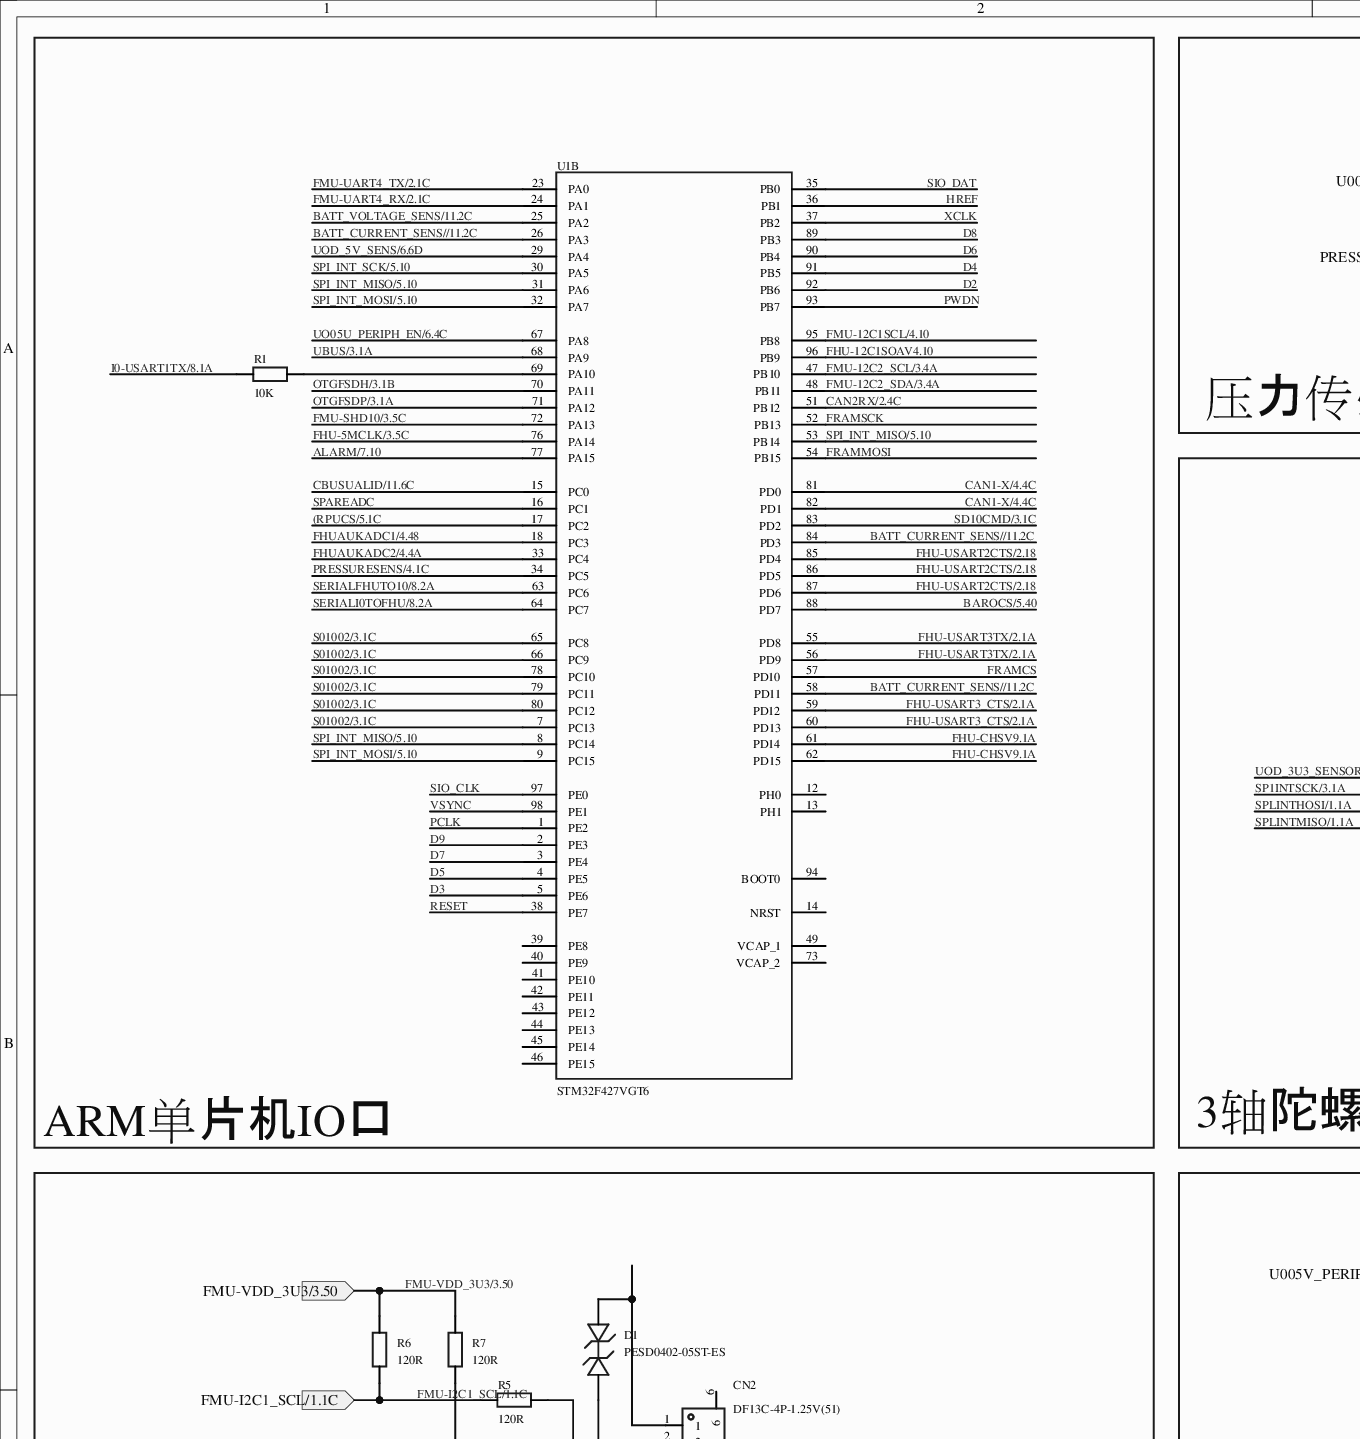
[diagram p0: MISC50255-3.schdoc, top left]
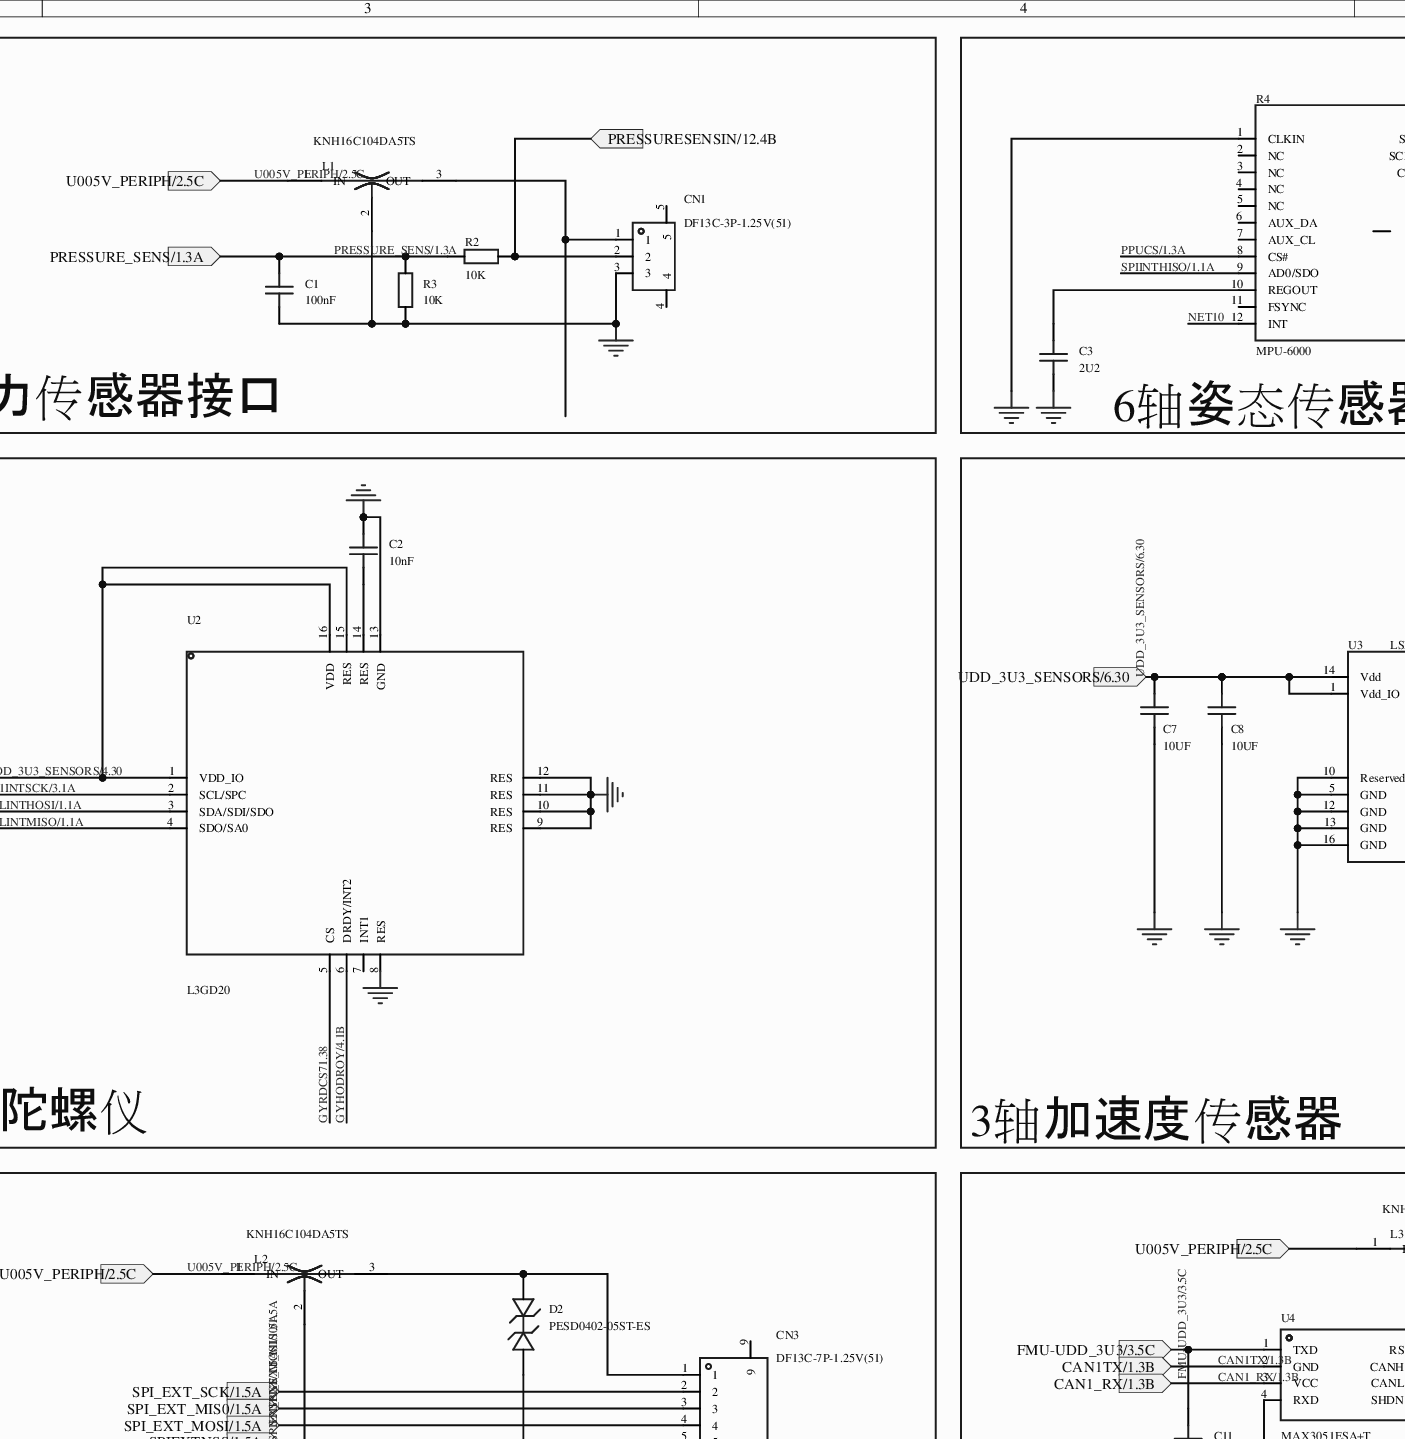
[diagram p1: MISC50255-3.schdoc, top middle]
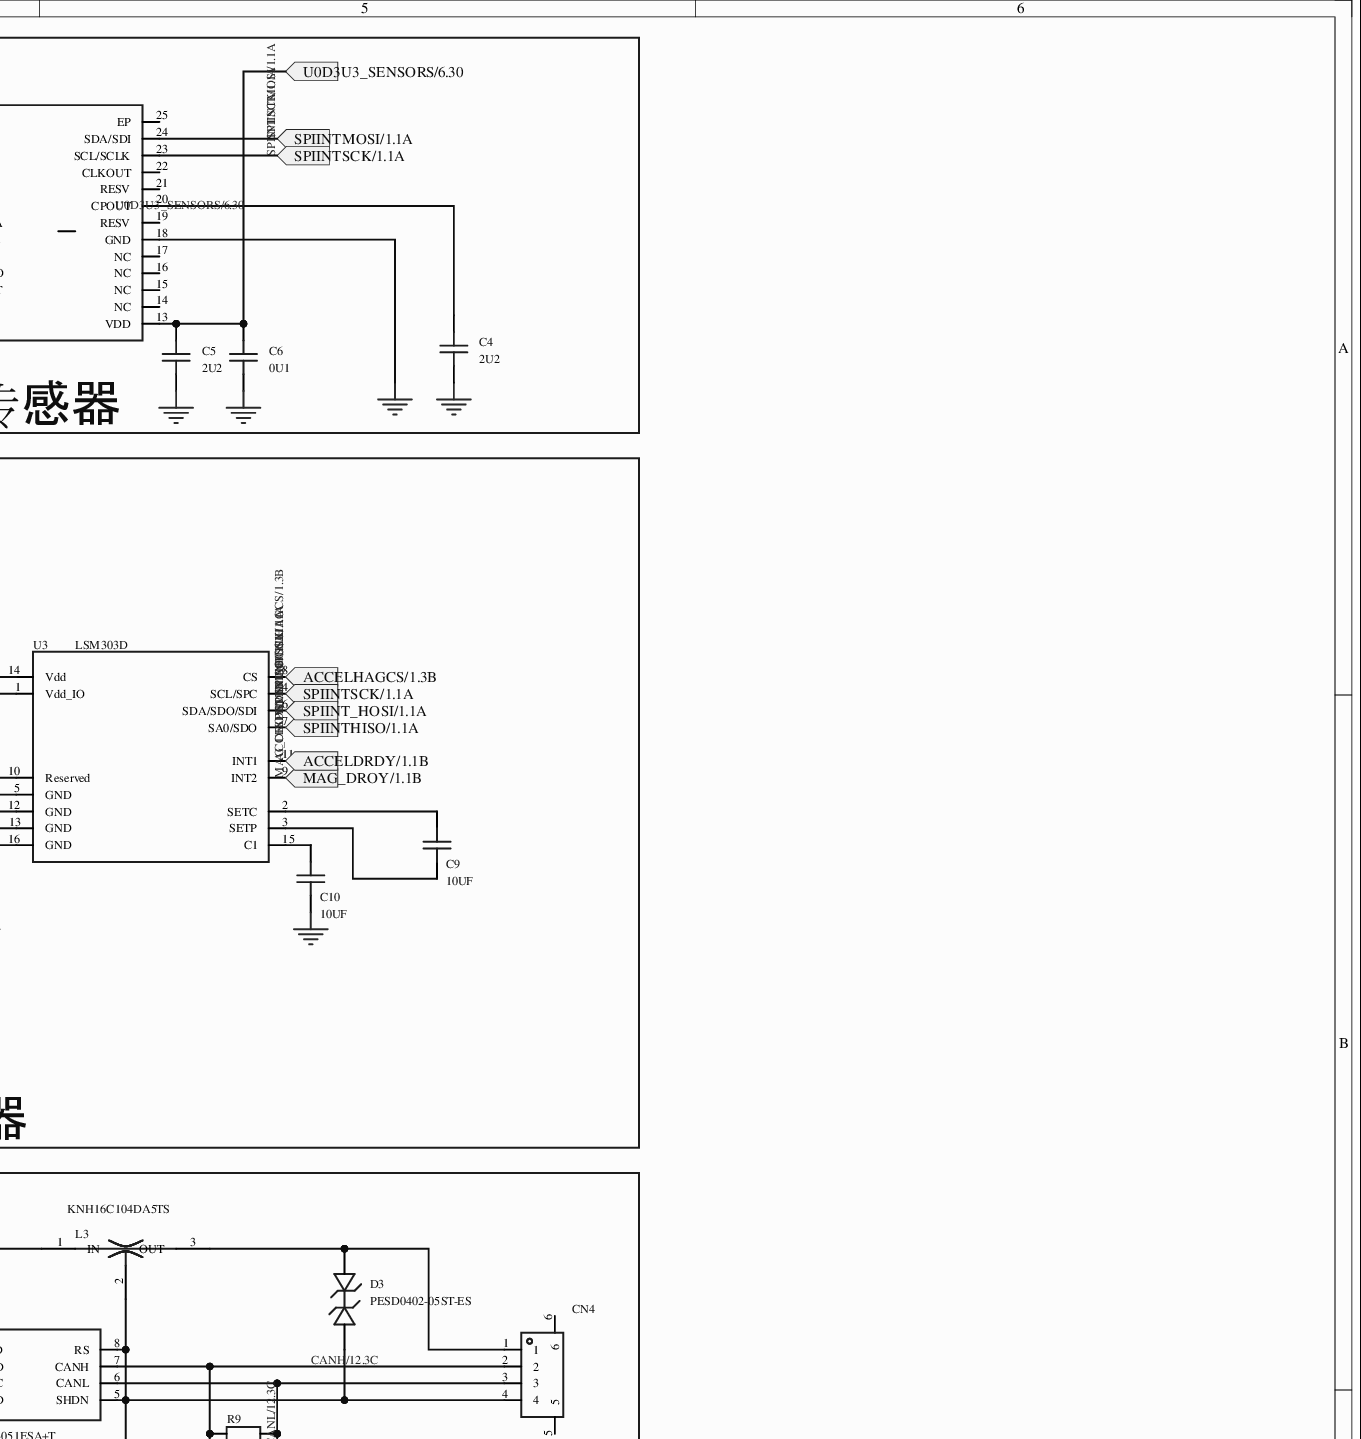
[diagram p2: MISC50255-3.schdoc, top right]
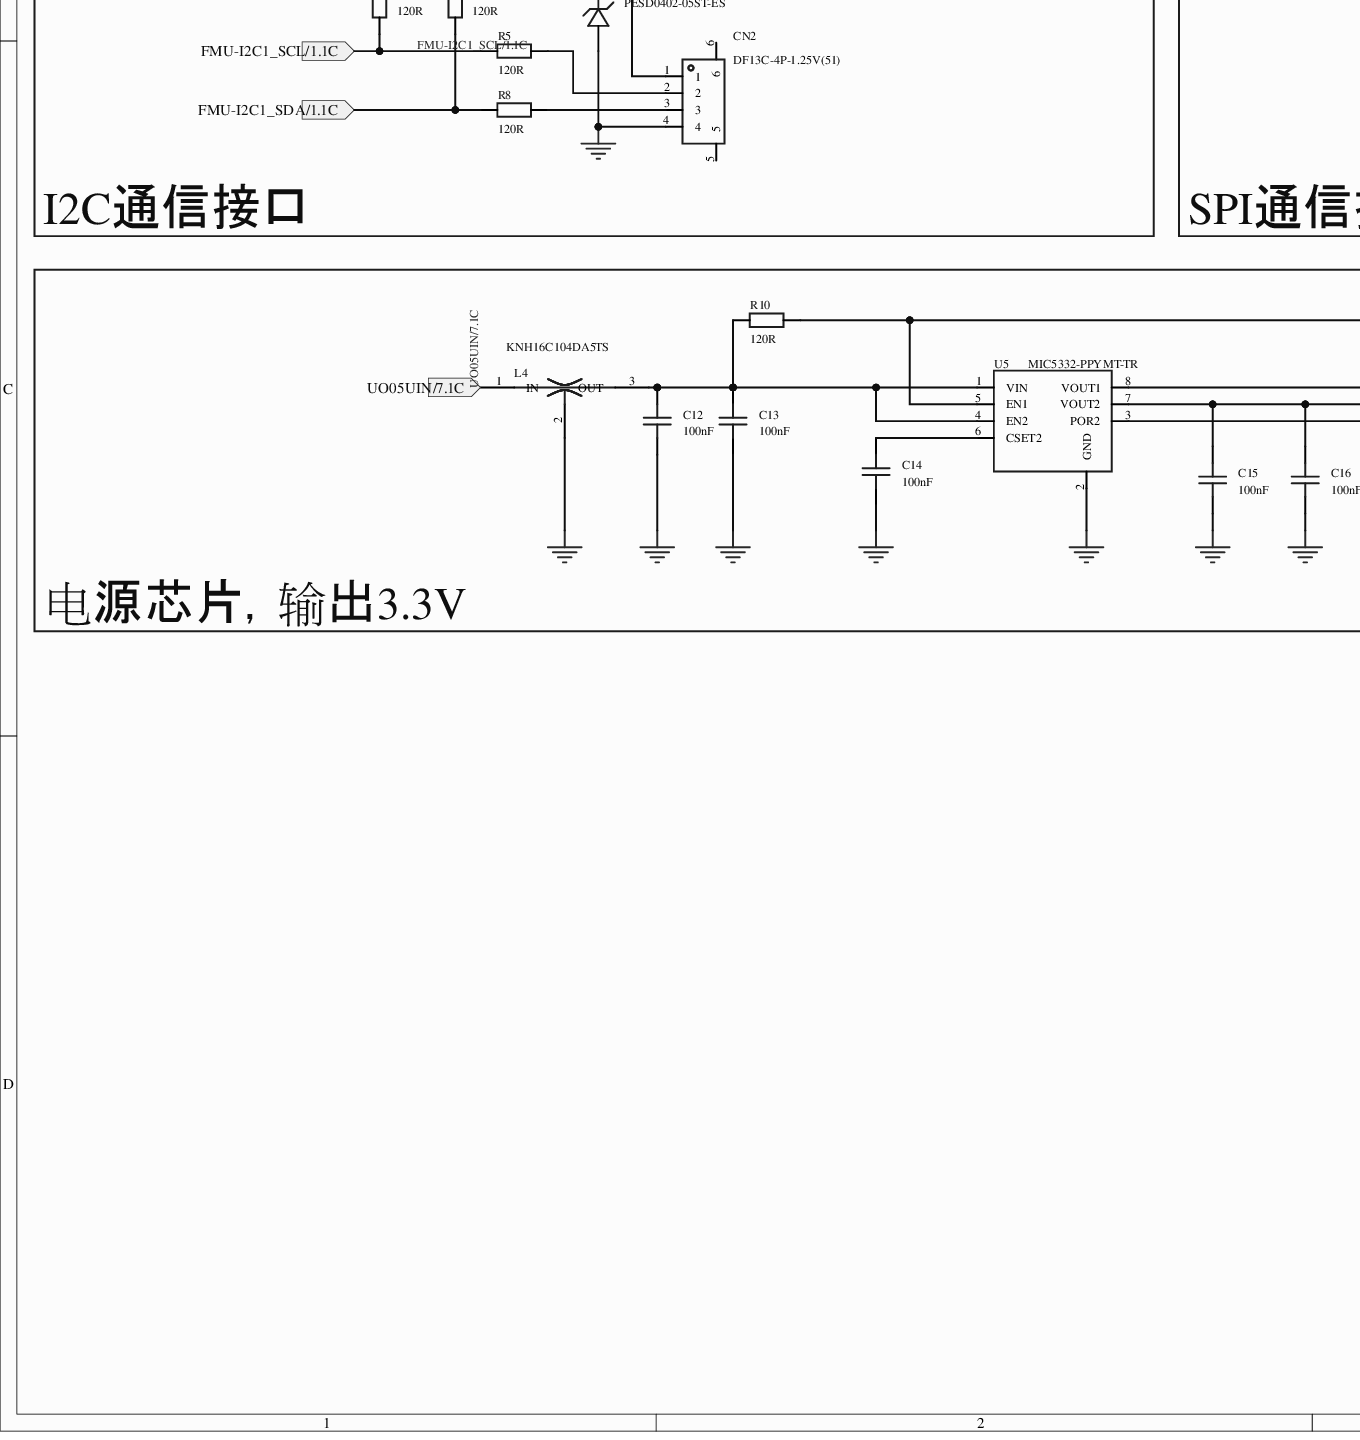
[diagram p3: MISC50255-3.schdoc, bottom left]
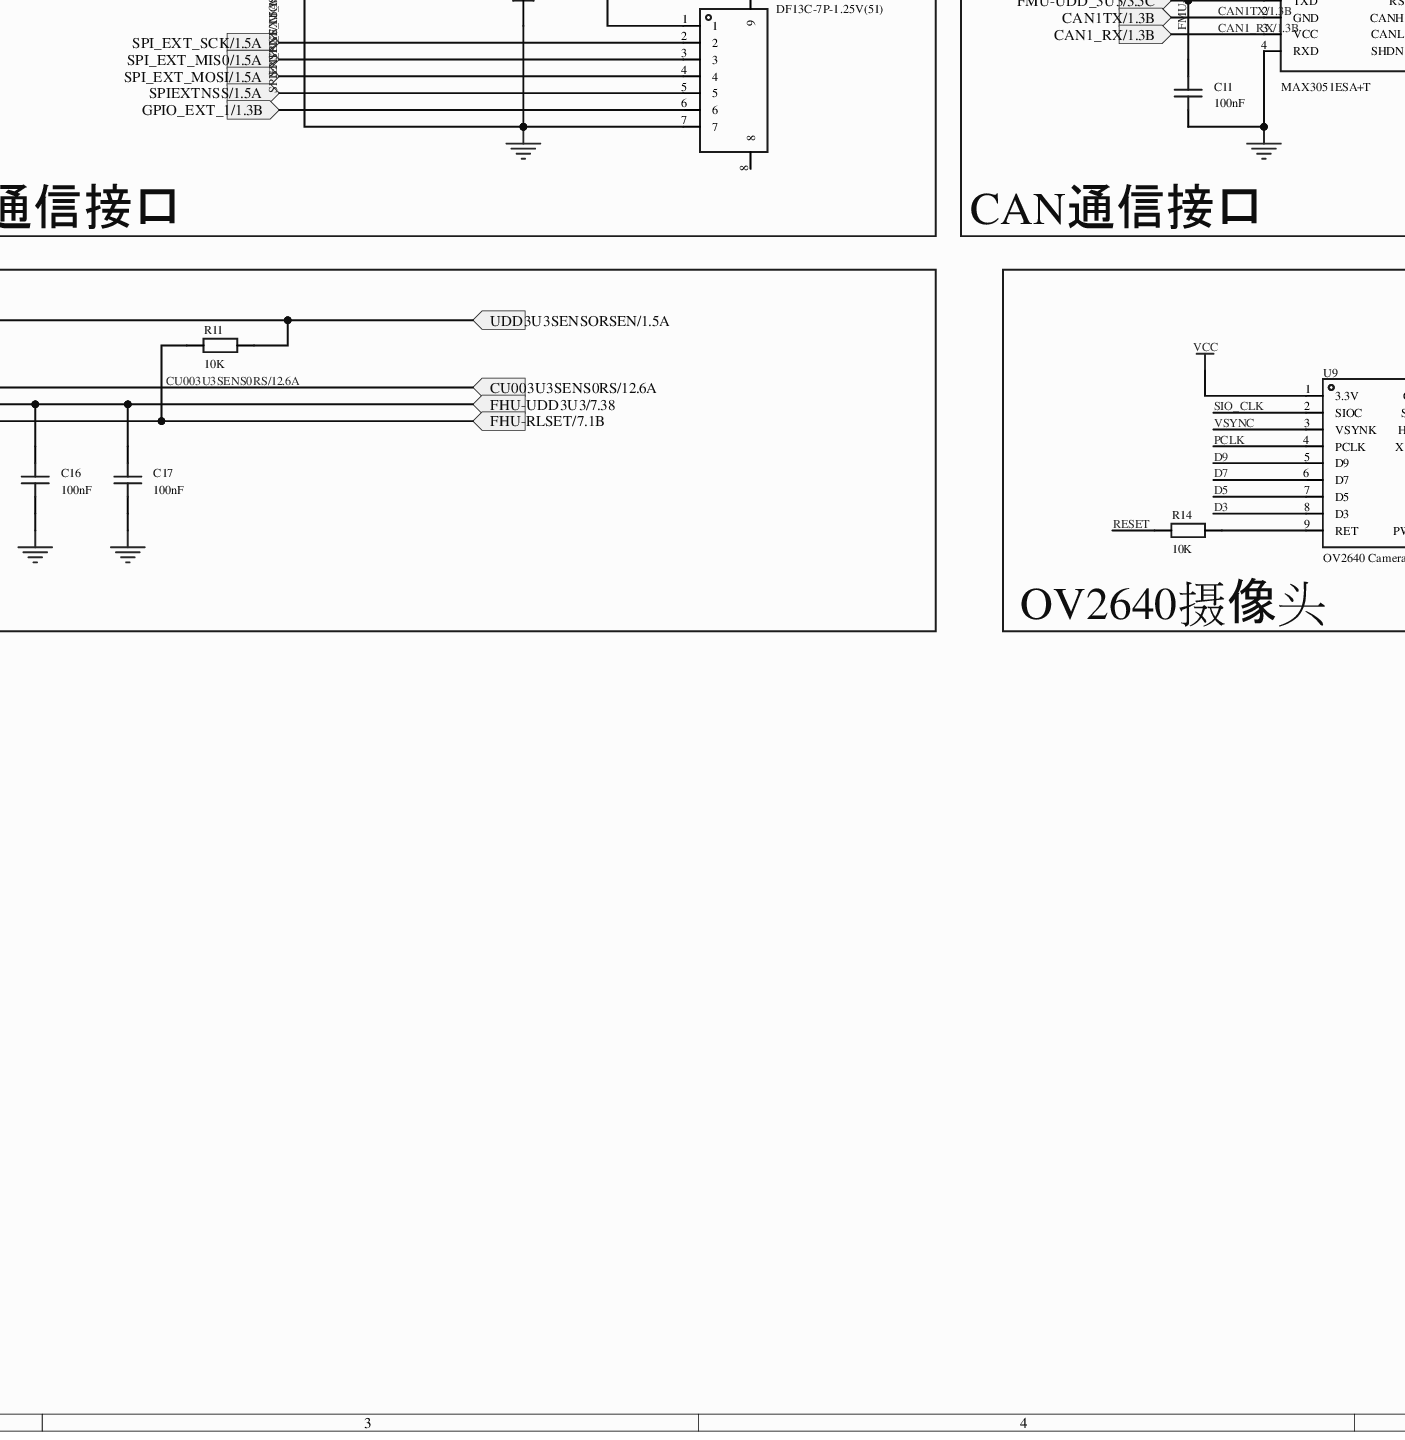
[diagram p4: MISC50255-3.schdoc, bottom middle]
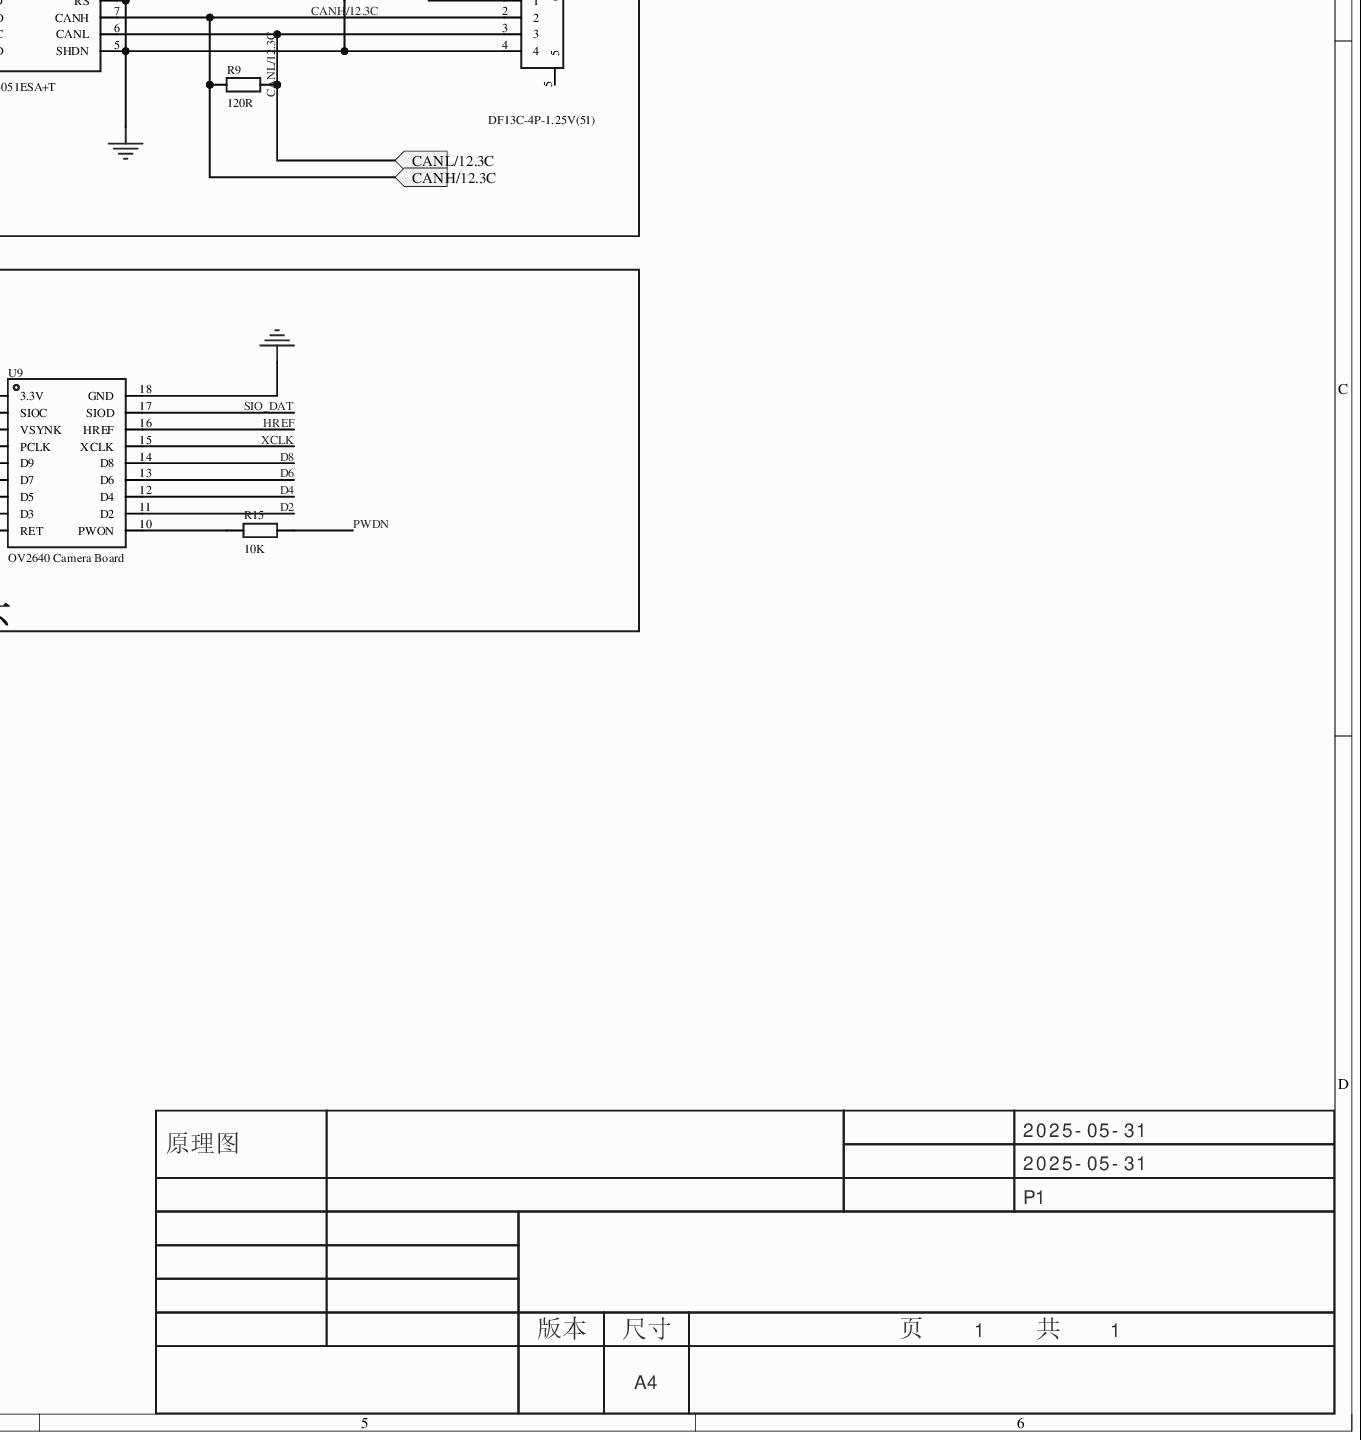
[diagram p5: MISC50255-3.schdoc, bottom right]
# Altium project MISC50255-2.PrjPcb
1 sheet, 47 parts. Net scope: flat (ports and power ports of the same name join across sheets).
Board file: MISC50255.pcbdoc

## Sheet MISC50255-3.schdoc
size 594 x 419 mm; Version: V1.0; @Project Name: MISC50255; @Page Count: 1; @Update Date: 2025-05-31; @Create Date: 2025-05-31; @Schematic Name: MISC50255; @Page No: 1; @Create Time: 19:12:28; @Update Time: 19:12:33; @Board Name: MISC50255

### Parts
C1  100nF  [C0603]
C2  10nF  [C0603]
C3  2U2  [C0603]
C4  2U2  [C0603]
C5  2U2  [C0603]
C6  0U1  [C0603]
C7  10UF  [C0603]
C8  10UF  [C0603]
C9  10UF  [C0603]
C10  10UF  [C0603]
C11  100nF  [C0603]
C12  100nF  [C0603]
C13  100nF  [C0603]
C14  100nF  [C0603]
C15  100nF  [C0603]
C16  100nF  [C0603]
C17  100nF  [C0603]
CN1  DF13C-3P-1.25V(51)  [CONN-SMD_3P-P1.25_DF13C-3P-1.25V]
CN2  DF13C-4P-1.25V(51)  [CONN-SMD_4P-P1.25_DF13C-4P-1.25V]
CN3  DF13C-7P-1.25V(51)  [CONN-SMD_7P-P1.25_DF13C-7P-1.25V]
CN4  DF13C-4P-1.25V(51)  [CONN-SMD_4P-P1.25_DF13C-4P-1.25V]
D1  PESD0402-05ST-ES  [DFN1006-2L-BI]
D2  PESD0402-05ST-ES  [DFN1006-2L-BI]
D3  PESD0402-05ST-ES  [DFN1006-2L-BI]
L1  KNH16C104DA5TS  [FILTER-SMD_3P-L1.6-W0.8_YFF18PCXXXXXXX]
L2  KNH16C104DA5TS  [FILTER-SMD_3P-L1.6-W0.8_YFF18PCXXXXXXX]
L3  KNH16C104DA5TS  [FILTER-SMD_3P-L1.6-W0.8_YFF18PCXXXXXXX]
L4  KNH16C104DA5TS  [FILTER-SMD_3P-L1.6-W0.8_YFF18PCXXXXXXX]
R1  10K  [R0603]
R2  10K  [R0603]
R3  10K  [R0603]
R4  MPU-6000  [QFN-24_L4.0-W4.0-P0.50-BL-EP2.7]
R5  120R  [R0603]
R6  120R  [R0603]
R7  120R  [R0603]
R8  120R  [R0603]
R9  120R  [R0603]
R10  120R  [R0603]
R11  10K  [R0603]
R14  10K  [R0603]
R15  10K  [R0603]
U1  STM32F427VGT6  [LQFP-100_L14.0-W14.0-P0.50-LS16.0-BL]  (part B of 2)
U2  L3GD20  [LGA-16_L4.0-W4.0-P0.65-BL]
U3  LSM303D  [LGA-16_L3.0-W3.0-P0.50-TL]
U4  MAX3051ESA+T  [SOIC-8_L4.9-W3.9-P1.27-LS6.0-BL]
U5  MIC5332-PPYMT-TR  [MLF-8_L2.0-W2.0-P0.50-BL-EP]
U9  OV2640 Camera Board  [SENSORM-TH_L35.7-W3.9-OV2640]

### Blocks framed on the sheet
ARM单片机IO口: R1 U1
压力传感器接口: C1 CN1 L1 R2 R3
6轴姿态传感器: C3-C6 R4
3轴陀螺仪: C2 U2
3轴加速度传感器: C7-C10 U3
I2C通信接口: CN2 D1 R5-R8
SPI通信接口: CN3 D2 L2
CAN通信接口: C11 CN4 D3 L3 R9 U4
电源芯片，输出3.3V: C12-C17 L4 R10 R11 U5
OV2640摄像头: R14 R15 U9

### Ports
ACCELDRDY/1.1B (in), ACCELHAGCS/1.3B (in), CAN1_RX/1.3B (in), CAN1TX/1.3B (in), CANH/12.3C (in), CANL/12.3C (in), CU003U3SENS0RS/12.6A (in), FHU-RLSET/7.1B (in), FHU-UDD3U3/7.38 (in), FMU-I2C1_SCL/1.1C (in), FMU-I2C1_SDA/1.1C (in), FMU-UDD_3U3/3.5C (in), FMU-VDD_3U3/3.50 (in), GPIO_EXT_1/1.3B (in), MAG_DROY/1.1B (in), PRESSURE_SENS/1.3A (in), PRESSURESENSIN/12.4B (in), SPI_EXT_MIS0/1.5A (in), SPI_EXT_MOSI/1.5A (in), SPI_EXT_SCK/1.5A (in), SPIEXTNSS/1.5A (in), SPIINT_HOSI/1.1A (in), SPIINTHISO/1.1A (in), SPIINTMOSI/1.1A (in), SPIINTSCK/1.1A (in), U0D3U3_SENSORS/6.30 (in), U005V_PERIPH/2.5C (in), UDD3U3SENSORSEN/1.5A (in), UDD_3U3_SENSORS/6.30 (in), UO05UIN/7.1C (in)

### Nets
GND: C1.1 C2.2 C3.1 C4.1 C5.1 C6.1 C7.1 C8.1 C10.1 C11.1 C12.1 C13.1 C14.1 C15.1 C16.1 C17.1 CN1.3 CN2.4 CN3.7 CN4.4 D1.1 D2.1 D3.1 L1.2(GND) L2.2(GND) L3.2(GND) L4.2(GND) R3.1 R4.1(CLKIN) R4.18(GND) U2.8(RES) U2.9(RES) U2.10(RES) U2.11(RES) U2.12(RES) U2.13(GND) U3.5(GND) U3.10(Reserved) U3.12(GND) U3.13(GND) U3.16(GND) U4.4(RXD) U4.5(SHDN) U4.8(RS) U5.2(GND) U9.18(GND)
VCC: U9.1(3.3V)
(RPUCS/5.1C: U1.17(PC2)
ACCELDRDY/1.1B: U3.11(INT1) ; port ACCELDRDY/1.1B
ACCELHAGCS/1.3B: U3.8(CS) ; port ACCELHAGCS/1.3B
ALARM/7.10: U1.77(PA15)
BAROCS/5.40: U1.88(PD7)
BATT_CURRENT_SENS//11.2C: U1.26(PA3) U1.58(PD11) U1.84(PD3)
BATT_VOLTAGE_SENS/11.2C: U1.25(PA2)
CAN1-X/4.4C: U1.81(PD0) U1.82(PD1)
CAN1_RX/1.3B: U4.3(VCC) ; port CAN1_RX/1.3B
CAN1TX/1.3B: U4.2(GND) ; port CAN1TX/1.3B
CAN2RX/2.4C: U1.51(PB12)
CANH/12.3C: CN4.2 R9.1 U4.7(CANH) ; port CANH/12.3C
CANL/12.3C: CN4.3 R9.2 U4.6(CANL) ; port CANL/12.3C
CBUSUALID/11.6C: U1.15(PC0)
CU003U3SENS0RS/12.6A: U5.8(VOUT1) ; port CU003U3SENS0RS/12.6A
D2: U1.92(PB6) U9.11(D2)
D3: U1.5(PE6) U9.8(D3)
D4: U1.91(PB5) U9.12(D4)
D5: U1.4(PE5) U9.7(D5)
D6: U1.90(PB4) U9.13(D6)
D7: U1.3(PE4) U9.6(D7)
D8: U1.89(PB3) U9.14(D8)
D9: U1.2(PE3) U9.5(D9)
FHU-5MCLK/3.5C: U1.76(PA14)
FHU-12C1SOAV4.10: U1.96(PB9)
FHU-CHSV9.1A: U1.61(PD14) U1.62(PD15)
FHU-USART2CTS/2.18: U1.85(PD4) U1.86(PD5) U1.87(PD6)
FHU-USART3_CTS/2.1A: U1.59(PD12) U1.60(PD13)
FHU-USART3TX/2.1A: U1.55(PD8) U1.56(PD9)
FHUAUKADC1/4.48: U1.18(PC3)
FHUAUKADC2/4.4A: U1.33(PC4)
FMU-12C1SCL/4.10: U1.95(PB8)
FMU-12C2_SCL/3.4A: U1.47(PB10)
FMU-12C2_SDA/3.4A: U1.48(PB11)
FMU-I2C1_SCL/1.1C: R5.1 R6.1 ; port FMU-I2C1_SCL/1.1C
FMU-SHD10/3.5C: U1.72(PA13)
FMU-UART4_RX/2.1C: U1.24(PA1)
FMU-UART4_TX/2.1C: U1.23(PA0)
FMU-UDD_3U3/3.5C: C11.2 U4.1(TXD) ; port FMU-UDD_3U3/3.5C
FMU-VDD_3U3/3.50: R6.2 R7.2 ; port FMU-VDD_3U3/3.50
FRAMCS: U1.57(PD10)
FRAMMOSI: U1.54(PB15)
FRAMSCK: U1.52(PB13)
GYHODROY/4.1B: U2.6(DRDY/INT2)
GYRDCS71.38: U2.5(CS)
HREF: U1.36(PB1) U9.16(HREF)
I0-USART1TX/8.1A: R1.1
MAG_DROY/1.1B: U3.9(INT2) ; port MAG_DROY/1.1B
NET10: R4.12(INT)
OTGFSDH/3.1B: U1.70(PA11)
OTGFSDP/3.1A: U1.71(PA12)
PCLK: U1.1(PE2) U9.4(PCLK)
PPUCS/1.3A: R4.8(CS#)
PRESSURE_SENS/1.3A: C1.2 R2.1 R3.2 ; port PRESSURE_SENS/1.3A
PRESSURESENS/4.1C: U1.34(PC5)
PWDN: R15.2 U1.93(PB7)
RESET: R14.1 U1.38(PE7)
S01002/3.1C: U1.7(PC13) U1.65(PC8) U1.66(PC9) U1.78(PC10) U1.79(PC11) U1.80(PC12)
SD10CMD/3.1C: U1.83(PD2)
SERIALFHUTO10/8.2A: U1.63(PC6)
SERIALI0TOFHU/8.2A: U1.64(PC7)
SIO_CLK: U1.97(PE0) U9.2(SIOC)
SIO_DAT: U1.35(PB0) U9.17(SIOD)
SP1INTSCK/3.1A: U2.2(SCL/SPC)
SPAREADC: U1.16(PC1)
SPI_EXT_MIS0/1.5A: CN3.3 ; port SPI_EXT_MIS0/1.5A
SPI_EXT_MOSI/1.5A: CN3.4 ; port SPI_EXT_MOSI/1.5A
SPI_INT_MISO/5.10: U1.8(PC14) U1.31(PA6) U1.53(PB14)
SPI_INT_MOSI/5.10: U1.9(PC15) U1.32(PA7)
SPI_INT_SCK/5.10: U1.30(PA5)
SPIEXTNSS/1.5A: CN3.5 ; port SPIEXTNSS/1.5A
SPIINT_HOSI/1.1A: U3.6(SDA/SDO/SDI) ; port SPIINT_HOSI/1.1A
SPIINTHISO/1.1A: R4.9(AD0/SDO) U3.7(SA0/SDO) ; port SPIINTHISO/1.1A
SPIINTMOSI/1.1A: R4.24(SDA/SDI) ; port SPIINTMOSI/1.1A
SPIINTSCK/1.1A: R4.23(SCL/SCLK) U3.4(SCL/SPC) ; port SPIINTSCK/1.1A
SPLINTHOSI/1.1A: U2.3(SDA/SDI/SDO)
SPLINTMISO/1.1A: U2.4(SDO/SA0)
U0D3U3_SENSORS/6.30: C5.2 C6.2 R4.13(VDD) ; port U0D3U3_SENSORS/6.30
U005V_PERIPH/2.5C: L1.1(IN) L2.1(IN) L3.1(IN) ; port U005V_PERIPH/2.5C
UBUS/3.1A: U1.68(PA9)
UDD_3U3_SENSORS/6.30: C7.2 C8.2 U3.1(Vdd_IO) U3.14(Vdd) ; port UDD_3U3_SENSORS/6.30
UO05U_PERIPH_EN/6.4C: U1.67(PA8)
UO05UIN/7.1C: L4.1(IN) ; port UO05UIN/7.1C
UOD_3U3_SENSORS/4.30: U2.1(VDD_IO) U2.15(RES) U2.16(VDD)
UOD_5V_SENS/6.6D: U1.29(PA4)
VSYNC: U1.98(PE1) U9.3(VSYNK)
XCLK: U1.37(PB2) U9.15(XCLK)
NetC2_1: C2.1 U2.14(RES)
NetC3_2: C3.2 R4.10(REGOUT)
NetC4_2: C4.2 R4.20(CPOUT)
NetC9_1: C9.1 U3.3(SETP)
NetC9_2: C9.2 U3.2(SETC)
NetC10_2: C10.2 U3.15(C1)
NetC12_2: C12.2 C13.2 L4.3(OUT) R10.1 U5.1(VIN) U5.4(EN2)
NetC14_2: C14.2 U5.6(CSET2)
NetC15_2: C15.2 C16.2 C17.2 U5.7(VOUT2) ; port FHU-UDD3U3/7.38
NetCN1_1: CN1.1 L1.3(OUT)
NetCN1_2: CN1.2 R2.2 ; port PRESSURESENSIN/12.4B
NetCN2_1: CN2.1 D1.2
NetCN2_2: CN2.2 R5.2
NetCN2_3: CN2.3 R8.2
NetCN3_1: CN3.1 D2.2 L2.3(OUT)
NetCN3_2: CN3.2 ; port SPI_EXT_SCK/1.5A
NetCN3_6: CN3.6 ; port GPIO_EXT_1/1.3B
NetCN4_1: CN4.1 D3.2 L3.3(OUT)
NetR1_2: R1.2 U1.69(PA10)
NetR7_1: R7.1 R8.1 ; port FMU-I2C1_SDA/1.1C
NetR10_2: R10.2 R11.2 U5.5(EN1) ; port UDD3U3SENSORSEN/1.5A
NetR11_1: R11.1 U5.3(POR2) ; port FHU-RLSET/7.1B
NetR14_2: R14.2 U9.9(RET)
NetR15_1: R15.1 U9.10(PWON)

Not connected (* = marked no-connect by the designer): CN1 4 5; CN2 5 6; CN3 8 9; CN4 5 6; R4 2 3(NC) 4(NC) 5(NC) 6(AUX_DA) 7(AUX_CL) 11(FSYNC) 14(NC) 15(NC) 16(NC) 17(NC) 19(RESV) 21(RESV) 22(CLKOUT) 25(EP); U1 12(PH0) 13(PH1) 14(NRST) 39(PE8) 40(PE9) 41(PE10) 42(PE11) 43(PE12) 44(PE13) 45(PE14) 46(PE15) 49(VCAP_1) 73(VCAP_2) 94(BOOT0); U2 7(INT1)*

### Notes on the sheet
- 2025-05-31
- 原理图
- P1
- 版本
- 尺寸
- A4
- 页    1    共    1

### Library data of the parts
C1-C17 = CAP_0603: ConvertToPcb: yes; SymbolName: CapAcitance; ModelId: ac125912035d415993ca9572d50418b1; ModelName: C0603_L1.6-W0.8-H0.8; ModelTransform: 62.992,31.496,0,0,0,0,0,0,0; Device: CAP_0603; AddInBom: yes; Supplier Footprint: 0603; FootprintName: C0603
  C1 C11-C17: Value: 100nF
  C2: Value: 10nF
  C3-C5: Value: 2U2
  C6: Value: 0U1
  C7-C10: Value: 10UF
CN1 = DF13C-3P-1.25V(51): 安装方式:立贴;排数:1;触头材质:黄铜;工作温度范围:-35℃~+85℃;; Manufacturer: HRS(广濑); AddInBom: yes; ModelId: da88e83e6191495cae5f6ea5f4f68194; ModelName: CONN-SMD_DF13C-P1.25-LS-3P; ModelTransform: 330.708,192.913,0,0,0,0,0,-23.622,0; Symbol: DF13C-3P-1.25V(51); Device: DF13C-3P-1.25V(51); LCSC Part Name: DF13C-3P-1.25V(51); SupplierPart: C17295747; ManufacturerPart: DF13C-3P-1.25V(51); Supplier Footprint: SMD; JLCPCB Part Class: 扩展库; Datasheet: https://atta.szlcsc.com/upload/public/pdf/source/20240705/7C20181FDC70388559B7C11F30890F4A.pdf; Supplier: LCSC; ConvertToPcb: yes; FootprintName: CONN-SMD_3P-P1.25_DF13C-3P-1.25V; Mounting Style: 立贴; Number of Rows: 1; Contact Material: 黄铜; Operating Temperature Range: -35℃~+85℃
CN2 CN4 = DF13C-4P-1.25V(51): 插针结构:1x4P;间距:1.25mm;安装方式:立贴;参考系列:-;总PIN数:4P;排数:1;每排PIN数:4;行距:-;额定电流:1A;触头材质:黄铜;工作温度范围:-35℃~+85℃;; Manufacturer: HRS(广濑); AddInBom: yes; ModelId: d6a5b94d17f346d5bcaafed7e659328c; ModelName: CONN-SMD_DF13C-P1.25-LS-4P; ModelTransform: 379.9205,192.913,0,0,0,0,-0.004,-21.654,0; Pins Structure: 1x4P; Pitch: 1.25mm; Number of PINs Per Row: 4; Current Rating (Max): 1A; Symbol: DF13C-4P-1.25V(51); Device: DF13C-4P-1.25V(51); LCSC Part Name: 1x4P 间距:1.25mm 立贴; SupplierPart: C531047; ManufacturerPart: DF13C-4P-1.25V(51); Supplier Footprint: SMD,P=1.25mm; JLCPCB Part Class: 扩展库; Datasheet: https://atta.szlcsc.com/upload/public/pdf/source/20200515/C531047_40B253F83E23310DAE4582CFE29D35CF.pdf; Supplier: LCSC; ConvertToPcb: yes; FootprintName: CONN-SMD_4P-P1.25_DF13C-4P-1.25V; Mounting Style: 立贴; Reference Series: -; Number of Pins: 4P; Number of Rows: 1; Row Spacing: -; Contact Material: 黄铜; Operating Temperature Range: -35℃~+85℃
CN3 = DF13C-7P-1.25V(51): 安装方式:立贴;排数:1;触头材质:黄铜;工作温度:-35℃~+85℃;; Manufacturer: HRS(广濑); AddInBom: yes; ModelId: b97e28e43dde4eb4a0341278d71f6c4f; ModelName: CONN-SMD_DF13C-P1.25-LS-7P; ModelTransform: 527.558,192.913,0,0,0,0,0,-15.118,0; Symbol: DF13C-7P-1.25V(51); Device: DF13C-7P-1.25V(51); LCSC Part Name: DF13C-7P-1.25V(51); SupplierPart: C17505353; ManufacturerPart: DF13C-7P-1.25V(51); Supplier Footprint: SMD; Datasheet: https://atta.szlcsc.com/upload/public/pdf/source/20240705/7C20181FDC70388559B7C11F30890F4A.pdf; Supplier: LCSC; ConvertToPcb: yes; FootprintName: CONN-SMD_7P-P1.25_DF13C-7P-1.25V; Mounting Type: 立贴; Number of Rows: 1; Contact Material: 黄铜; Operating Temperature: -35℃~+85℃
D1-D3 = PESD0402-05ST-ES: 极性:双向;反向截止电压(Vrwm):5V;最大钳位电压:25V;峰值脉冲电流(Ipp):4.5A;峰值脉冲功率(Ppp):120W;击穿电压:9V;; Manufacturer: ElecSuper(静芯微); AddInBom: yes; ModelId: 2bdbcca3b35b49c5a8ae725a08658930; ModelTransform: 40.1574,24.4094,0,0,0,0,0,0,0; polarity: 双向; Reverse Stand-Off Voltage (Vrwm): 5V; Maximum Clamping Voltage: 25V; Peak Pulse Current (Ipp): 4.5A; Peak Pulse Power Dissipation (Ppp): 120W; Breakdown Voltage: 9V; Reverse Leakage Current (Ir): 1uA; Number of Lines: 单路; Type: ESD; Junction Capacitance: 0.25pF; Symbol: PESD0402-05ST-ES; Device: PESD0402-05ST-ES; LCSC Part Name: PESD0402-05ST-ES; SupplierPart: C41409253; ManufacturerPart: PESD0402-05ST-ES; Supplier Footprint: DFN1006-2L; JLCPCB Part Class: 扩展库; Datasheet: https://atta.szlcsc.com/upload/public/pdf/source/20240918/8FBBEB995DF809C9DD42750341680481.pdf; Supplier: LCSC; ConvertToPcb: yes; FootprintName: DFN1006-2L-BI; ModelName: DFN1006-2L-BI; Operating Temperature: -40℃~+125℃; level of protection: -
L1-L4 = KNH16C104DA5TS_C7435624: AddInBom: yes; ModelId: 9d067bcebd9d43a2821eee12b9b96cab; ModelName: FILTER-SMD_3P-L1.6-W0.8-H0.6_YFF18PCXXXXXXX; ModelTransform: 63.7794,32.283,0,0,0,0,0,0,0; Symbol: KNH16C104DA5TS_C7435624; Device: KNH16C104DA5TS_C7435624; LCSC Part Name: KNH16C104DA5TS; SupplierPart: C7435624; ManufacturerPart: KNH16C104DA5TS; Supplier Footprint: 0603; JLCPCB Part Class: 扩展库; Supplier: LCSC; ConvertToPcb: yes; FootprintName: FILTER-SMD_3P-L1.6-W0.8_YFF18PCXXXXXXX
R1-R3 R5-R11 R14 R15 = Res_0603: ConvertToPcb: yes; SymbolName: 电阻; ModelId: fc143cca1e79419f9cd78b61e9279f08; ModelTransform: 31.8897,63.7794,0,90,0,0,0,0,0; Device: Res_0603; AddInBom: yes; Supplier Footprint: 0603; FootprintName: R0603; ModelName: R0603
  R1-R3 R11 R14 R15: Value: 10K
  R5-R10: Value: 120R
R4 = MPU-6000: 传感器类型:加速度计陀螺仪;; Manufacturer: TDK InvenSense(应美盛); AddInBom: yes; ModelId: 3147e748bde04e038f0f2a42301e4816; ModelTransform: 158.267,158.267,0,0,0,0,0,0,0; Symbol: MPU-6000; Device: MPU-6000; LCSC Part Name: MPU-6000; SupplierPart: C92401; ManufacturerPart: MPU-6000; Supplier Footprint: QFN-24-EP(4x4); Datasheet: https://atta.szlcsc.com/upload/public/pdf/source/20170418/1492506341548.pdf; Supplier: LCSC; ConvertToPcb: yes; FootprintName: QFN-24_L4.0-W4.0-P0.50-BL-EP2.7; ModelName: QFN-24_L4.0-W4.0-P0.50-BL-EP2.7; Sensor Type: 加速度计陀螺仪; Operating Temperature: -40℃~+85℃
U1 = STM32F427VGT6: CPU内核:ARM-M4;CPU最大主频:180MHz;应用领域:-;; Manufacturer: ST(意法半导体); Relevance: []; AddInBom: yes; ModelId: 469e6cc70557486dbd01fd12ff814964; ModelName: LQFP-100_L14.0-W14.0-H1.4-LS16.0-P0.50; ModelTransform: 629.92,629.92,0,0,0,0,0,0,0; CPU Core: ARM-M4; CPU Maximum Speed: 180MHz; Program Storage Size: 1MB; Program Memory Type: FLASH; Number of I/O: 82; ADC (Bit): 12bit; Low Voltage Detection Threshold: 1.8V~3.6V; Symbol: STM32F427VGT6; Device: STM32F427VGT6; LCSC Part Name: 带DSP和FPU的高性能高级系列ARM Cortex-M4 MCU，具有1 MB Flash、180 MHz CPU、ART加速器、Chrom-ART加速器和FSMC; SupplierPart: C117815; ManufacturerPart: STM32F427VGT6; Supplier Footprint: LQFP-100(14x14); JLCPCB Part Class: 扩展库; Datasheet: https://atta.szlcsc.com/upload/public/pdf/source/20171120/C75389_15111748895051131877.pdf; Supplier: LCSC; ConvertToPcb: yes; FootprintName: LQFP-100_L14.0-W14.0-P0.50-LS16.0-BL; DAC (Bit): 12bit; Application Area: -
U2 = L3GD20: 三轴芯片 陀螺仪 3轴 2000DPS 16LGA MEMS 传感器输出: 数字 测量轴: X, Y, Z 满量程率范围: ± 250°/s, ± 500°/s, ± 2000°/s 电源电压最小值: 2.4V 电源电压最大值: 3.6V 封装类型: LGA 针脚数: 16 灵敏度类型: 8.75m°/s/digit, 17.5m°/s/digit, 70m°/s/digit MSL: MSL 3 - 168小时 SVHC(高度关注物质): No SVHC (19-Dec-2012); Manufacturer: ST(意法半导体); AddInBom: yes; ModelId: 29d0564020bd43c6a1357a4861850bfc; ModelName: LGA-16_L4.0-W4.0-H1.1-P0.65; ModelTransform: 157.48,157.48,0,90,0,0,0,0,0; Symbol: L3GD20; Device: L3GD20; LCSC Part Name: L3GD20; SupplierPart: C15641; ManufacturerPart: L3GD20; Supplier Footprint: LGA-16(4x4); JLCPCB Part Class: 扩展库; Datasheet: https://atta.szlcsc.com/upload/public/pdf/source/20170925/C116866_1506321365621990121.pdf; Supplier: LCSC; ConvertToPcb: yes; FootprintName: LGA-16_L4.0-W4.0-P0.65-BL
U3 = LSM303D: AddInBom: yes; ModelId: 9ae441d1842848bda5fda48efd45bd94; ModelTransform: 118.11,118.11,0,0,0,0,0,0,0; Symbol: LSM303D; Device: LSM303D; LCSC Part Name: LSM303D; SupplierPart: C9900017210; ManufacturerPart: LSM303D; Supplier Footprint: LGA-16; Supplier: LCSC; ConvertToPcb: yes; FootprintName: LGA-16_L3.0-W3.0-P0.50-TL; ModelName: LGA-16_L3.0-W3.0-P0.50-TL
U4 = MAX3051ESA+T: 类型:CAN收发器;数据速率:1Mbps;; Manufacturer: ADI(亚德诺)/MAXIM(美信); AddInBom: yes; ModelId: e81d2f7d937b4a6ab1dca543ff5d56a4; ModelName: SOIC-8_L4.9-W3.9-H1.7-LS6.0-P1.27; ModelTransform: 189.751,236.22,0,0,0,0,0.0005,0.0005,0; Data Rate: 1Mbps; Supply Voltage: 3.3V; Supply Current: 35mA; Symbol: MAX3051ESA+T; Device: MAX3051ESA+T; LCSC Part Name: MAX3051 CAN收发器; SupplierPart: C15648; ManufacturerPart: MAX3051ESA+T; Supplier Footprint: SOIC-8; Datasheet: https://atta.szlcsc.com/upload/public/pdf/source/20130726/1457706626418.pdf; Supplier: LCSC; ConvertToPcb: yes; FootprintName: SOIC-8_L4.9-W3.9-P1.27-LS6.0-BL; Type: CAN收发器; Operating Temperature: -40℃~+85℃
U5 = MIC5332-PPYMT-TR: Manufacturer: MICROCHIP(美国微芯); AddInBom: yes; ModelId: 9e278931321a4d59b91dd471bba85e04; ModelTransform: 78.74,78.74,0,0,0,0,0.001,-0.001,0; Symbol: MIC5332-PPYMT-TR; Device: MIC5332-PPYMT-TR; LCSC Part Name: MIC5332-PPYMT-TR; SupplierPart: C622303; ManufacturerPart: MIC5332-PPYMT-TR; Supplier Footprint: MLF-8; Datasheet: https://atta.szlcsc.com/upload/public/pdf/source/20171228/C153276_15144475830431215029.pdf; Supplier: LCSC; ConvertToPcb: yes; FootprintName: MLF-8_L2.0-W2.0-P0.50-BL-EP; ModelName: MLF-8_L2.0-W2.0-P0.50-BL-EP
U9 = OV2640 Camera Board: 供电电压：3.3VIO电压：1.7V ~3.3V DC; Manufacturer: Waveshare(微雪电子); AddInBom: yes; Symbol: OV2640 CAMERA BOARD; Device: OV2640 Camera Board; LCSC Part Name: OV2640摄像头 OV2640模块 OV2640摄像头 采集模组 200万像素; SupplierPart: C359962; ManufacturerPart: OV2640 Camera Board; Supplier Footprint: -; JLCPCB Part Class: 扩展库; Datasheet: https://atta.szlcsc.com/upload/public/pdf/source/20190107/C359962_8F9E613A403684C90116CB7314EC2612.pdf; Supplier: LCSC; ConvertToPcb: yes; FootprintName: SENSORM-TH_L35.7-W3.9-OV2640